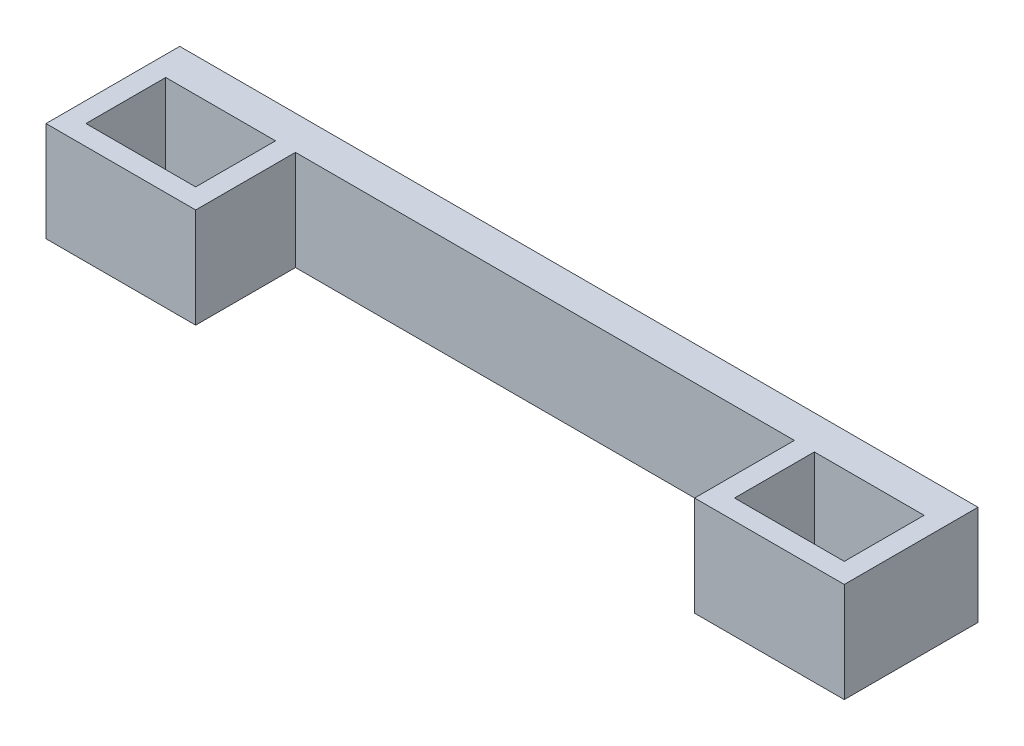
SolidWorks part; units mm, degrees
material "普通碳钢"
ref_plane "Front Plane" through (0, 0, 0) normal (0, 0, 1) x (1, 0, 0)
ref_plane "Top Plane" through (0, 0, 0) normal (0, 1, 0) x (1, 0, 0)
ref_plane "Right Plane" through (0, 0, 0) normal (1, 0, 0) x (0, 0, -1)
sketch "Sketch1" plane through (0, 0, 0) normal (0, 1, 0) x (1, 0, 0)
  line L1 (-400, -67) -> (400, -67)
  line L2 (-400, -67) -> (-400, 67)
  line L3 (-400, 67) -> (400, 67)
  line L4 (400, -67) -> (400, 67)
  line L5 (-400, -67) -> (400, 67) construction
  line L6 (-400, 67) -> (400, -67) construction
  point P0 (0, 0)
  dimension "D1" = 800
  dimension "D2" = 134
extrude "Boss-Extrude1" add sketch "Sketch1" along normal blind 100
sketch "Sketch2" plane through (0, 100, 0) normal (0, 1, 0) x (1, 0, 0)
  line L0 (0, 118.5785) -> (0, -216.9007) construction
  line L1 (-400, -67) -> (400, -67) construction
  line L2 (-250, -167) -> (250, -167)
  line L3 (-250, -167) -> (-250, 33)
  line L4 (-250, 33) -> (250, 33)
  line L5 (250, -167) -> (250, 33)
  line L6 (-250, -167) -> (250, 33) construction
  line L7 (-250, 33) -> (250, -167) construction
  point P3 (0, -67)
  dimension "D1" = 500
  dimension "D2" = 100
extrude "Cut-Extrude1" cut sketch "Sketch2" against normal blind 100
sketch "Sketch3" plane through (0, 100, 0) normal (0, 1, 0) x (1, 0, 0)
  line L0 (-421.3893, -47) -> (-231.1815, -47) construction
  line L1 (-400, -67) -> (-250, -67) construction
  line L2 (-380, 89.9583) -> (-380, -121.2692) construction
  line L3 (-400, 67) -> (-400, -67) construction
  line L4 (-250, 33) -> (-250, -67) construction
  line L5 (-380, -47) -> (-270, -47)
  line L6 (-380, -47) -> (-380, 33)
  line L7 (-380, 33) -> (-270, 33)
  line L8 (-270, -47) -> (-270, 33)
  dimension "D1" = 20
  dimension "D2" = 20
  dimension "D3" = 80
  dimension "D4" = 20
extrude "Cut-Extrude2" cut sketch "Sketch3" against normal blind 80
mirror "Mirror1" about plane through (0, 0, 0) normal (1, 0, 0) of "Cut-Extrude2"
split "Split2" [suppressed] bodies to split 104
split "Split3" [suppressed] bodies to split 108
split "Split4" [suppressed] bodies to split 110 111
